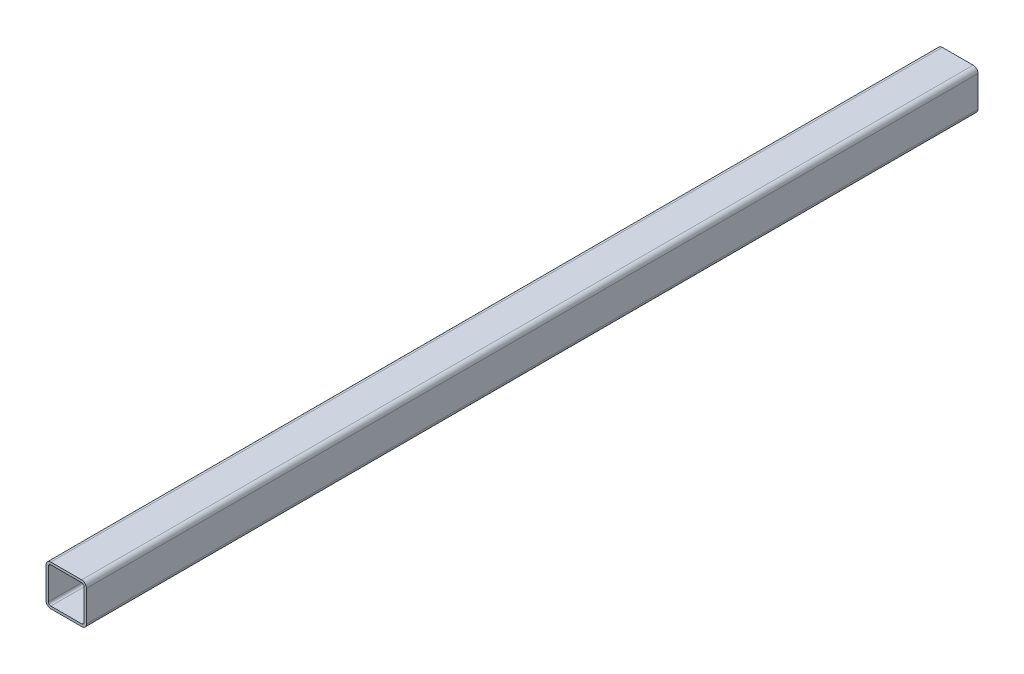
SolidWorks part; units mm, degrees
ref_plane "前视基准面" through (0, 0, 0) normal (0, 0, 1) x (1, 0, 0)
ref_plane "上视基准面" through (0, 0, 0) normal (0, 1, 0) x (1, 0, 0)
ref_plane "右视基准面" through (0, 0, 0) normal (1, 0, 0) x (0, 0, -1)
sketch "草图1" plane through (0, 0, 0) normal (0, 1, 0) x (1, 0, 0)
  line L0 (0, 0) -> (0, 1100)
  dimension "D1" = 1100
other "Gb／6728-1986方形空心型钢 050 X 50 X 3(1)"
ref_plane "基准面1" through (0, 0, 0) normal (0, 0, -1) x (-1, 0, 0)
sketch "Sketch1" plane through (0, 0, 0) normal (0, 0, -1) x (-1, 0, 0)
  line L0 (-19, -22) -> (19, -22)
  line L1 (-22, -19) -> (-22, 19)
  line L2 (19, 22) -> (-19, 22)
  line L3 (22, 19) -> (22, -19)
  line L4 (-19, -25) -> (19, -25)
  line L5 (-25, -19) -> (-25, 19)
  line L6 (19, 25) -> (-19, 25)
  line L7 (25, 19) -> (25, -19)
  arc A0 (25, 19) -> (19, 25) centre (19, 19) ccw
  arc A1 (19, -25) -> (25, -19) centre (19, -19) ccw
  arc A2 (-25, -19) -> (-19, -25) centre (-19, -19) ccw
  arc A3 (-19, 25) -> (-25, 19) centre (-19, 19) ccw
  arc A4 (-19, 22) -> (-22, 19) centre (-19, 19) ccw
  arc A5 (22, 19) -> (19, 22) centre (19, 19) ccw
  arc A6 (19, -22) -> (22, -19) centre (19, -19) ccw
  arc A7 (-22, -19) -> (-19, -22) centre (-19, -19) ccw
  point P0 (-25, 0)
  point P1 (25, 0)
  point P2 (0, 25)
  point P3 (0, -25)
  point P4 (0, 0)
  point P5 (-25, -25)
  point P6 (25, -25)
  point P7 (25, 25)
  point P8 (-25, 25)
  point P33 (0, 0)
  dimension "D1" = 6
  dimension "Thickness" = 3
  dimension "V_leg" = 50
